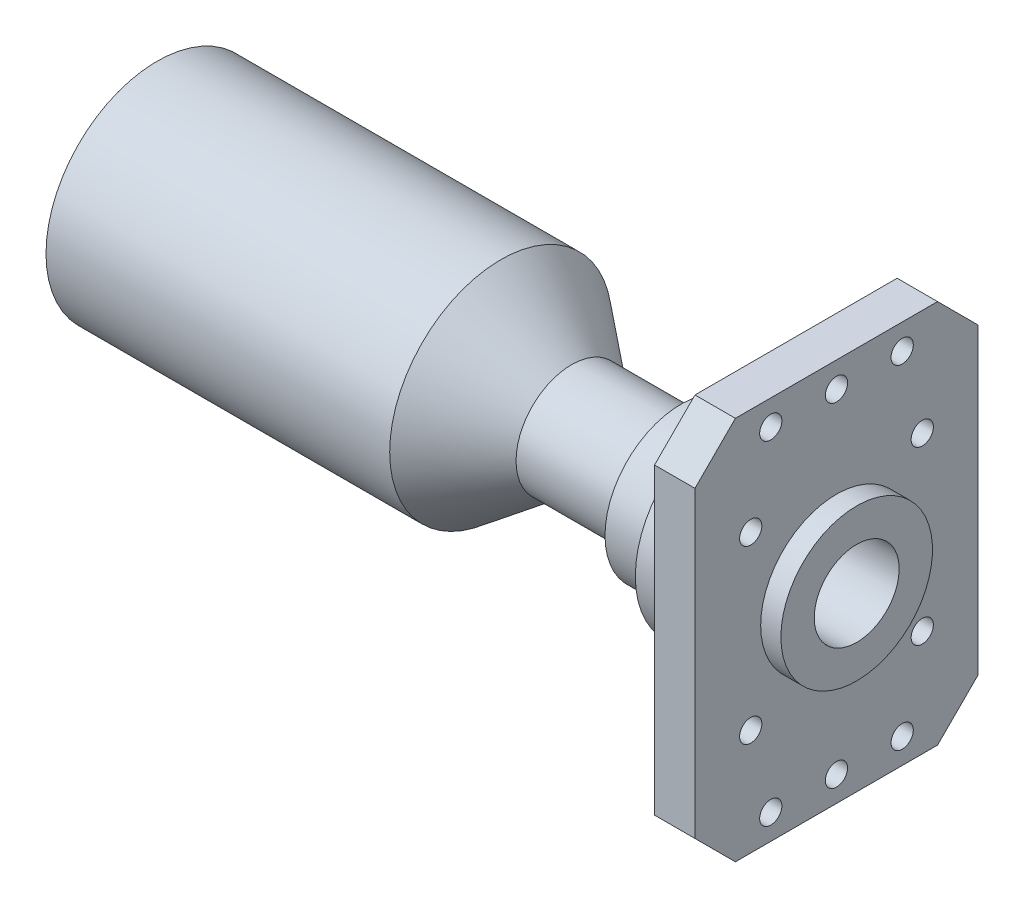
SolidWorks part; units mm, degrees
ref_plane "前视基准面" through (0, 0, 0) normal (0, 0, 1) x (1, 0, 0)
ref_plane "上视基准面" through (0, 0, 0) normal (0, 1, 0) x (1, 0, 0)
ref_plane "右视基准面" through (0, 0, 0) normal (1, 0, 0) x (0, 0, -1)
sketch "草图1" plane through (0, 0, 0) normal (0, 0, 1) x (1, 0, 0)
  line L0 (-107.8, 0) -> (112.4444, 0) construction
  line L1 (106.2222, -21) -> (56.2222, -21)
  line L2 (56.2222, -21) -> (56.2222, -17.5)
  line L3 (56.2222, -17.5) -> (-239.7778, -17.5)
  line L4 (-239.7778, -17.5) -> (-239.7778, -30)
  line L5 (-224.7778, -32.5) -> (-204.7778, -32.5)
  line L6 (-204.7778, -32.5) -> (-204.7778, -35)
  line L7 (-204.7778, -35) -> (-194.7778, -35)
  line L8 (-194.7778, -35) -> (-187.2778, -27.5)
  line L9 (19.2222, -27.5) -> (-187.2778, -27.5)
  line L10 (19.2222, -27.5) -> (19.2222, -37.5)
  line L11 (19.2222, -37.5) -> (44.2222, -37.5)
  line L12 (44.2222, -37.5) -> (44.2222, -47.5)
  line L13 (44.2222, -47.5) -> (64.2222, -47.5)
  line L14 (64.2222, -47.5) -> (76.2222, -68.5)
  line L15 (76.2222, -68.5) -> (76.2222, -95)
  line L16 (76.2222, -95) -> (96.2222, -95)
  line L17 (96.2222, -95) -> (96.2222, -37.5)
  line L18 (96.2222, -37.5) -> (106.2222, -37.5)
  line L19 (106.2222, -37.5) -> (106.2222, -21)
  line L20 (-239.7778, -30) -> (-224.7778, -30)
  line L21 (-224.7778, -30) -> (-224.7778, -32.5)
  dimension "D2" = 50
  dimension "D3" = 3.5
  dimension "D4" = 21
  dimension "D5" = 296
  dimension "D6" = 12.5
  dimension "D7" = 17.5
  dimension "D8" = 2.5
  dimension "D9" = 10
  dimension "D10" = 206.5
  dimension "D11" = 57.5
  dimension "D12" = 10
  dimension "D13" = 20
  dimension "D14" = 26.5
  dimension "D15" = 20
  dimension "D16" = 25
  dimension "D17" = 12
  dimension "D18" = 10
  dimension "D19" = 10
  dimension "D20" = 16.5
  dimension "D21" = 21
  dimension "D22" = 20
  dimension "D23" = 15
revolve "旋转1" add sketch "草图1" angle 360 about L0
sketch "草图2" plane through (96.2222, 0, 0) normal (1, 0, 0) x (0, 0, -1)
  line L2 (70, -64.2738) -> (70, 64.2738)
  line L4 (-70, -64.2738) -> (-70, 64.2738)
  arc A0 (70, -64.2738) -> (70, 64.2738) centre (0, 0) ccw
  arc A1 (-70, 64.2738) -> (-70, -64.2738) centre (0, 0) ccw
  point P0 (0, 0)
extrude "切除-拉伸1" cut sketch "草图2" against normal up to next
sketch "草图3" plane through (96.2222, 0, 0) normal (1, 0, 0) x (0, 0, -1)
  line L0 (-70, 64.2262) -> (70, 64.2262)
  line L1 (50, -95) -> (-50, -95)
  line L2 (70, -75) -> (70, -64.2262)
  line L3 (50, 95) -> (-50, 95)
  line L4 (-70, -75) -> (-70, -64.2262)
  line L5 (70, -95) -> (-70, 95) construction
  line L6 (70, 95) -> (-70, -95) construction
  line L7 (70, -64.2262) -> (-70, -64.2262)
  line L8 (-70, 64.2262) -> (-70, 75)
  line L9 (70, 64.2262) -> (70, 75)
  line L10 (70, 75) -> (50, 95)
  line L11 (-50, 95) -> (-70, 75)
  line L12 (-50, -95) -> (-70, -75)
  line L13 (50, -95) -> (70, -75)
  point P0 (0, 0)
extrude "凸台-拉伸2" add sketch "草图3" against normal up to surface (20 mm away) contours L3 L11 L8 L0 L9 L10
sketch "草图4" plane through (96.2222, 0, 0) normal (1, 0, 0) x (0, 0, -1)
  line L1 (-120.7218, 0) -> (159.7552, 0) construction
  line L2 (0, 102.0099) -> (0, -110.8628) construction
  line L3 (0, -110.8628) -> (4.8289, -104.4243) construction
  line L4 (50, 95) -> (-50, 95) construction
  circle A0 centre (42.4264, 42.4264) radius 5.5
  circle A1 centre (42.4264, -42.4264) radius 5.5
  circle A2 centre (-42.4264, -42.4264) radius 5.5
  circle A3 centre (-42.4264, 42.4264) radius 5.5
  circle A4 centre (0, 82.5) radius 5.5
  circle A5 centre (-32.5, 82.5) radius 5.5
  circle A6 centre (32.5, 82.5) radius 5.5
  circle A7 centre (32.5, -82.5) radius 5.5
  circle A8 centre (0, -82.5) radius 5.5
  circle A9 centre (-32.5, -82.5) radius 5.5
  point P19 (0, 0)
  dimension "D3" = 11
  dimension "D1" = 11
  dimension "D5" = 11
  dimension "D6" = 11
  dimension "D7" = 32.5
  dimension "D8" = 32.5
  dimension "D9" = 12.5
  dimension "D4" = 4
extrude "切除-拉伸2" cut sketch "草图4" against normal up to next contours A0
sketch "草图5" plane through (-239.7778, 0, 0) normal (-1, 0, 0) x (0, 0, 1)
  circle A0 centre (0, 0) radius 42.5
  circle A1 centre (0, 0) radius 55
  dimension "D1" = 85
  dimension "D2" = 110
extrude "凸台-拉伸3" add sketch "草图5" against normal blind 170 separate body
ref_axis "基准轴1" through (-69.7778, 0, 0) along (-1, 0, 0)
sketch "草图7" plane through (0, 0, 0) normal (0, 0, 1) x (1, 0, 0)
  line L0 (-69.7778, 55) -> (-69.7778, 27.5)
  line L1 (19.2222, 27.5) -> (-187.2778, 27.5) construction
  line L2 (-69.7778, -55) -> (-69.7778, 55) construction
  line L3 (-69.7778, 27.5) -> (-34.7778, 27.5)
  line L4 (-34.7778, 27.5) -> (-69.7778, 55)
  dimension "D1" = 35
revolve "旋转2" add sketch "草图7" angle 360 about axis through (-69.7778, 0, 0) along (-1, 0, 0)
sketch "草图8" plane through (-239.7778, 0, 0) normal (-1, 0, 0) x (0, 0, 1)
  circle A0 centre (0, 0) radius 35
extrude "切除-拉伸3" cut sketch "草图8" against normal blind 175
sketch "草图9" plane through (0, 0, 0) normal (0, 0, 1) x (1, 0, 0)
  line L0 (-69.7778, 0) -> (-239.7778, 0) construction
  line L1 (-224.7778, 11) -> (-89.7778, 11)
  line L3 (-224.7778, -11) -> (-89.7778, -11)
  line L5 (-224.7778, 11) -> (-89.7778, -11) construction
  line L6 (-224.7778, -11) -> (-89.7778, 11) construction
  line L8 (-239.7778, 55) -> (-239.7778, -55) construction
  arc A0 (-224.7778, 11) -> (-224.7778, -11) centre (-224.7778, 0) ccw
  arc A1 (-89.7778, 11) -> (-89.7778, -11) centre (-89.7778, 0) cw
  point P0 (-157.2778, 0)
  dimension "D3" = 15
  dimension "D1" = 135
  dimension "D2" = 22
extrude "切除-拉伸4" cut sketch "草图9" against normal mid plane 95
